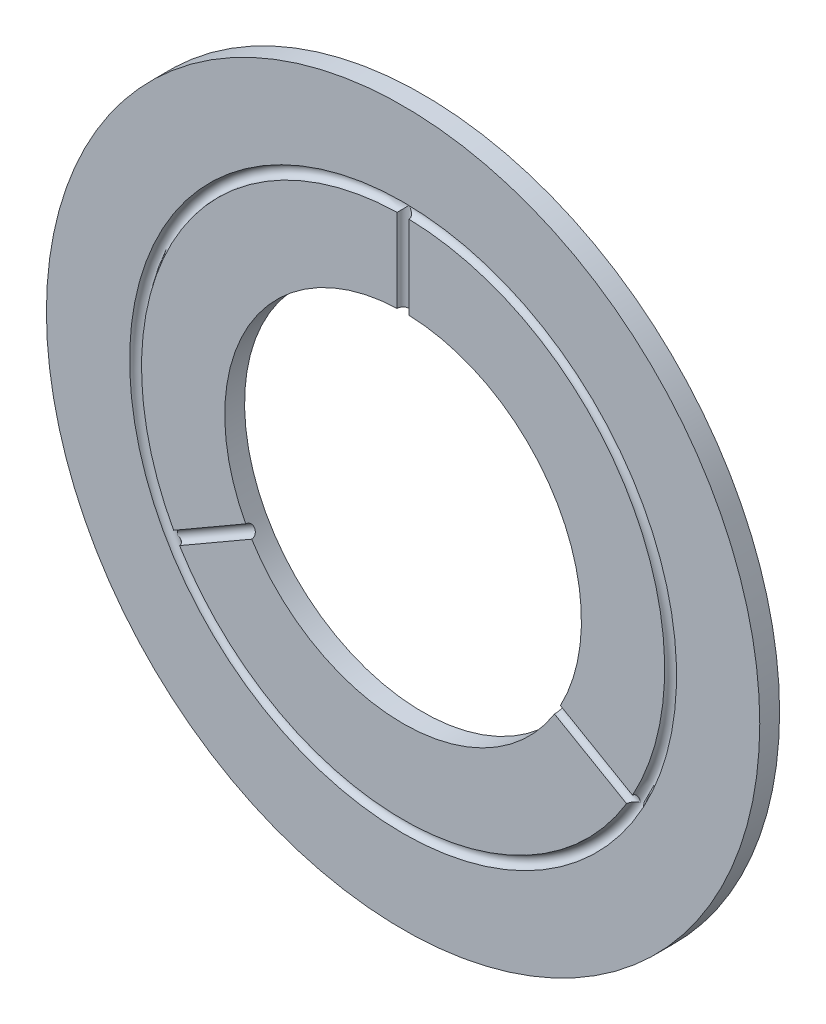
SolidWorks part; units mm, degrees
material "黄铜"
ref_plane "前视基准面" through (0, 0, 0) normal (0, 0, 1) x (1, 0, 0)
ref_plane "上视基准面" through (0, 0, 0) normal (0, 1, 0) x (1, 0, 0)
ref_plane "右视基准面" through (0, 0, 0) normal (1, 0, 0) x (0, 0, -1)
sketch "草图1" plane through (0, 0, 0) normal (0, 0, 1) x (1, 0, 0)
  circle A0 centre (0, 0) radius 45
  circle A1 centre (0, 0) radius 90
  dimension "D1" = 90
  dimension "D2" = 180
extrude "凸台-拉伸1" add sketch "草图1" along normal blind 5
sketch "草图2" plane through (0, 0, 5) normal (0, 0, 1) x (1, 0, 0)
  circle A0 centre (0, 0) radius 67.5
  dimension "D1" = 135
sketch "草图3" plane through (0, 0, 0) normal (1, 0, 0) x (0, 0, -1)
  line L0 (-5, 67.5) -> (-5, -67.5) construction
  line L1 (-5, 90) -> (-5, -90) construction
  line L2 (-5, 67.5) -> (-5, 0) construction
  circle A0 centre (-5, 67.5) radius 1.5
  dimension "D1" = 3
  dimension "D2" = 67.5
sweep "切除-扫描1" cut profiles "草图3" path "草图2"
sketch "草图5" plane through (0, 0, 0) normal (0, 1, 0) x (1, 0, 0)
  line L0 (-90, -5) -> (90, -5) construction
  circle A0 centre (0, -5) radius 1.5
  dimension "D1" = 3
extrude "切除-拉伸2" cut sketch "草图5" along normal blind 67.5
pattern_circular "阵列(圆周)1" count 3 over 360 about axis through (0, 0, 5) along (0, 0, -1) of "切除-拉伸2"
